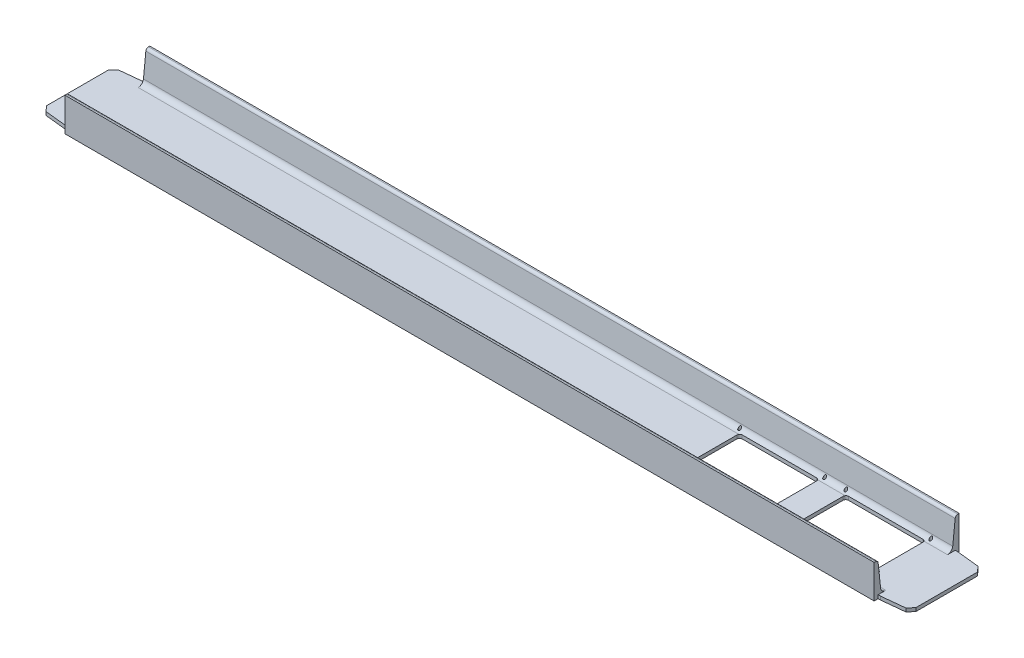
from build123d import *

# Parameters (mm, degrees)
GBT706_2008_16A_1_DEPTH = 1637
CUT_EXTRUDE_1_DEPTH     = 837.367891541
CUT_EXTRUDE_2_DEPTH     = 837.367891541
SKETCH_4_W              = 56.5
SKETCH_4_H              = 56.5
CUT_EXTRUDE_3_DEPTH     = 835.965313439
SKETCH_5_W              = 56.5
SKETCH_5_H              = 56.5
CUT_EXTRUDE_4_DEPTH     = 835.965313439
CUT_EXTRUDE_5_REACH     = 838.368
HOLE_WIZARD_M6_1_D      = 5


with BuildPart() as part:
    # Sketch12 → Gbt706-2008 热轧槽钢 16A(1) (new body)
    with BuildSketch(Plane.YZ.offset(-818.5)):
        with BuildLine():
            Line((63, 160), (0, 160))
            Line((0, 160), (0, 0))
            Line((0, 0), (63, 0))
            Line((63, 0), (63, 2.528785132))
            ThreePointArc((63, 2.528785132), (61.715724127, 5.874438164), (58.522642316, 7.501394609))
            Line((58.522642316, 7.501394609), (15.454715367, 12.028016136))
            ThreePointArc((15.454715367, 12.028016136), (9.068551745, 15.281929026), (6.5, 21.973235089))
            Line((6.5, 21.973235089), (6.5, 138.026764911))
            ThreePointArc((6.5, 138.026764911), (9.068551745, 144.718070974), (15.454715367, 147.971983864))
            Line((15.454715367, 147.971983864), (58.522642316, 152.498605391))
            ThreePointArc((58.522642316, 152.498605391), (61.715724127, 154.125561836), (63, 157.471214868))
            Line((63, 157.471214868), (63, 160))
        make_face()
    extrude(amount=GBT706_2008_16A_1_DEPTH)

    # 草图2 → 切除-拉伸1 (cut, through all)
    with BuildSketch(Plane.XZ):
        Polygon((762, -5), (762, 7.501394609), (766.477357684, 7.501394609), (809.545284633, 12.028016136), (818.5, 21.973235089), (818.5, 138.026764911), (809.545284633, 147.971983864), (766.477357684, 152.498605391), (762, 152.498605391), (762, 165), (828.5, 165), (828.5, -5), align=None)
    extrude(amount=-CUT_EXTRUDE_1_DEPTH, mode=Mode.SUBTRACT)

    # 草图3 → 切除-拉伸2 (cut, through all)
    with BuildSketch(Plane.XZ):
        Polygon((-762, 0), (-762, 7.501394609), (-766.477357684, 7.501394609), (-809.545284633, 12.028016136), (-818.5, 21.973235089), (-818.5, 138.026764911), (-809.545284633, 147.971983864), (-766.477357684, 152.498605391), (-762, 152.498605391), (-762, 165), (-838.5, 165), (-838.5, -5), (-762, -5), align=None)
    extrude(amount=-CUT_EXTRUDE_2_DEPTH, mode=Mode.SUBTRACT)

    # 草图4 → 切除-拉伸3 (cut, through all)
    with BuildSketch(Plane.XY.offset(152.498605391)):
        with Locations((790.25, 34.75)):
            Rectangle(SKETCH_4_W, SKETCH_4_H)
    extrude(amount=-CUT_EXTRUDE_3_DEPTH, mode=Mode.SUBTRACT)

    # 草图5 → 切除-拉伸4 (cut, through all)
    with BuildSketch(Plane.XY.offset(152.498605391)):
        with Locations((-790.25, 34.75)):
            Rectangle(SKETCH_5_W, SKETCH_5_H)
    extrude(amount=-CUT_EXTRUDE_4_DEPTH, mode=Mode.SUBTRACT)

    # 草图6 → 切除-拉伸5 (cut, up to next)
    with BuildSketch(Plane.XZ, mode=Mode.PRIVATE) as cut_extrude_5_sk1:
        with BuildLine():
            Line((513.5, 20), (373.5, 20))
            ThreePointArc((373.5, 20), (369.964466094, 21.464466094), (368.5, 25))
            Line((368.5, 25), (368.5, 105))
            ThreePointArc((368.5, 105), (369.964466094, 108.535533906), (373.5, 110))
            Line((373.5, 110), (513.5, 110))
            ThreePointArc((513.5, 110), (517.035533906, 108.535533906), (518.5, 105))
            Line((518.5, 105), (518.5, 25))
            ThreePointArc((518.5, 25), (517.035533906, 21.464466094), (513.5, 20))
        make_face()
    cut_extrude_5_tool1 = extrude(cut_extrude_5_sk1.sketch, amount=-CUT_EXTRUDE_5_REACH, mode=Mode.PRIVATE) & part.part
    # 草图6 → 切除-拉伸5 (cut, up to next)
    with BuildSketch(Plane.XZ, mode=Mode.PRIVATE) as cut_extrude_5_sk2:
        with BuildLine():
            Line((718.5, 25), (718.5, 105))
            ThreePointArc((718.5, 105), (717.035533906, 108.535533906), (713.5, 110))
            Line((713.5, 110), (573.5, 110))
            ThreePointArc((573.5, 110), (569.964466094, 108.535533906), (568.5, 105))
            Line((568.5, 105), (568.5, 25))
            ThreePointArc((568.5, 25), (569.964466094, 21.464466094), (573.5, 20))
            Line((573.5, 20), (713.5, 20))
            ThreePointArc((713.5, 20), (717.035533906, 21.464466094), (718.5, 25))
        make_face()
    cut_extrude_5_tool2 = extrude(cut_extrude_5_sk2.sketch, amount=-CUT_EXTRUDE_5_REACH, mode=Mode.PRIVATE) & part.part
    add(cut_extrude_5_tool1.solids().sort_by_distance((443.5, 0, 65))[0], mode=Mode.SUBTRACT)
    add(cut_extrude_5_tool2.solids().sort_by_distance((643.5, 0, 65))[0], mode=Mode.SUBTRACT)

    # M6 螺纹孔1 (through all)
    with Locations(Plane(origin=(0, 0, 0), x_dir=(-1, 0, 0), z_dir=(0, -1, 0))):
        with Locations((-723.5, -15), (-523.5, -15), (-563.5, -15), (-363.5, -15), (-563.5, -115), (-363.5, -115), (-723.5, -115), (-523.5, -115)):
            Hole(HOLE_WIZARD_M6_1_D / 2)


solid = part.part
